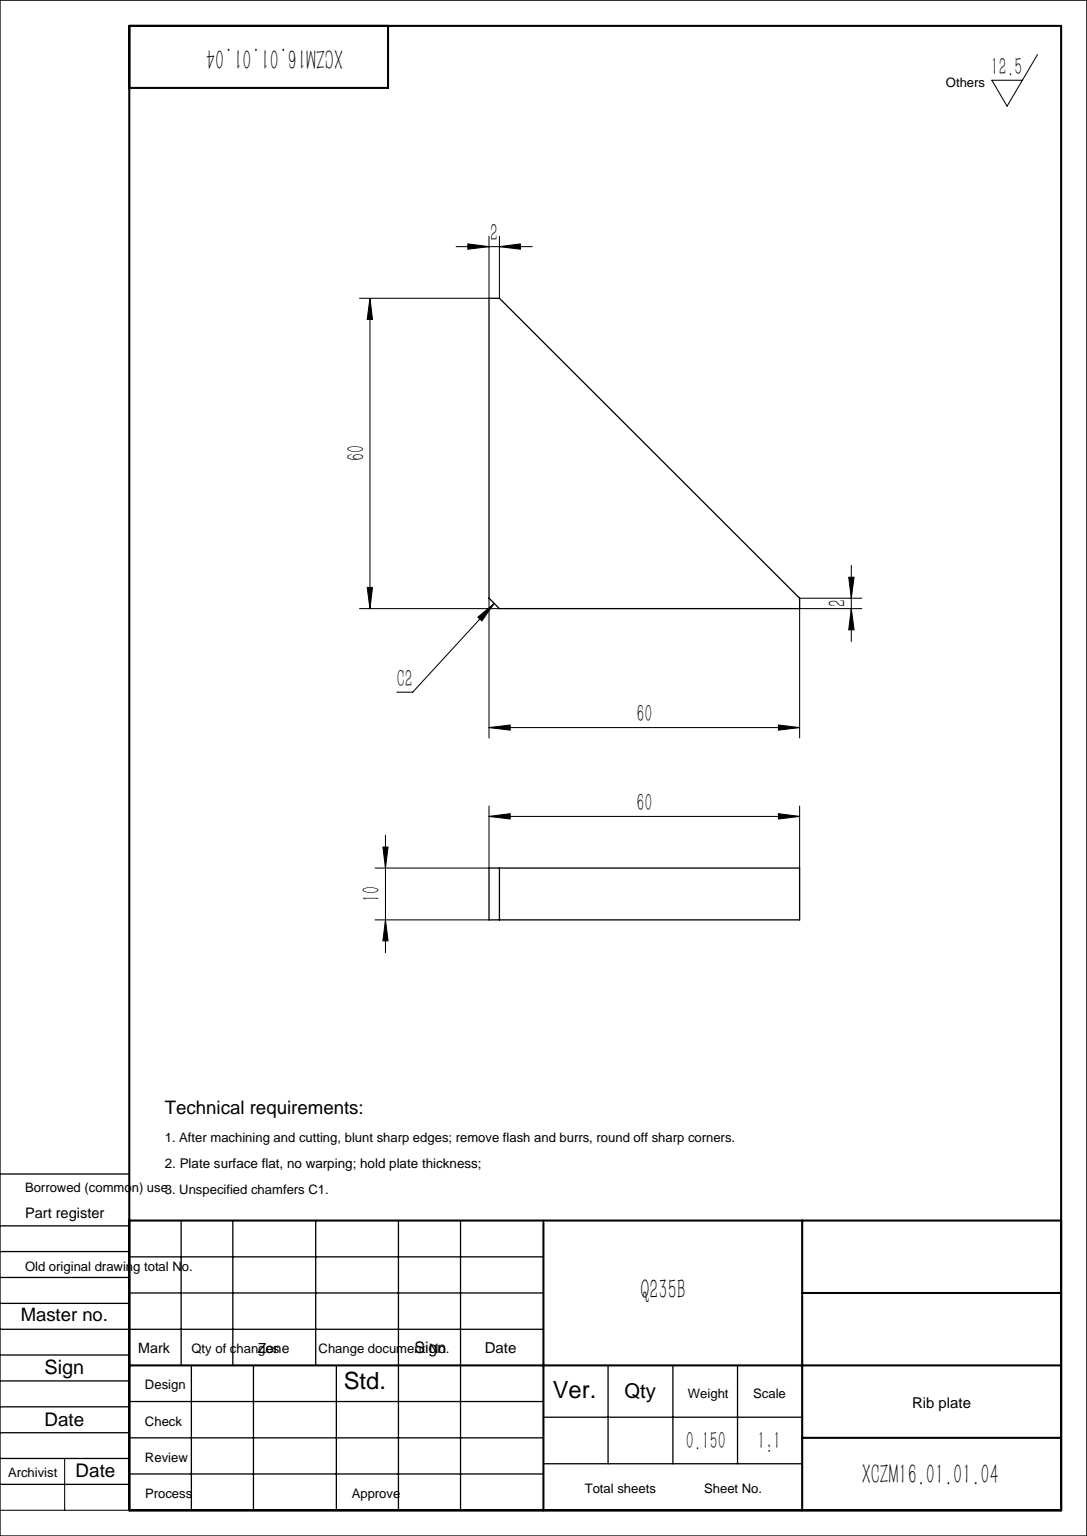
from build123d import *

# Parameters (mm, degrees)
BOSS_EXTRUDE1_DEPTH = 10
CHAMFER1_SIZE       = 2


with BuildPart() as part:
    # Sketch1 → Boss-Extrude1 (new body)
    with BuildSketch(Plane.XY):
        Polygon((0, 60), (0, 0), (60, 0), (60, 2), (2, 60), align=None)
    extrude(amount=BOSS_EXTRUDE1_DEPTH)

    # Chamfer1
    chamfer1_edges = [part.edges().sort_by_distance(p)[0] for p in [
        (0, 0, 5),
    ]]
    chamfer(chamfer1_edges, length=CHAMFER1_SIZE)


solid = part.part
